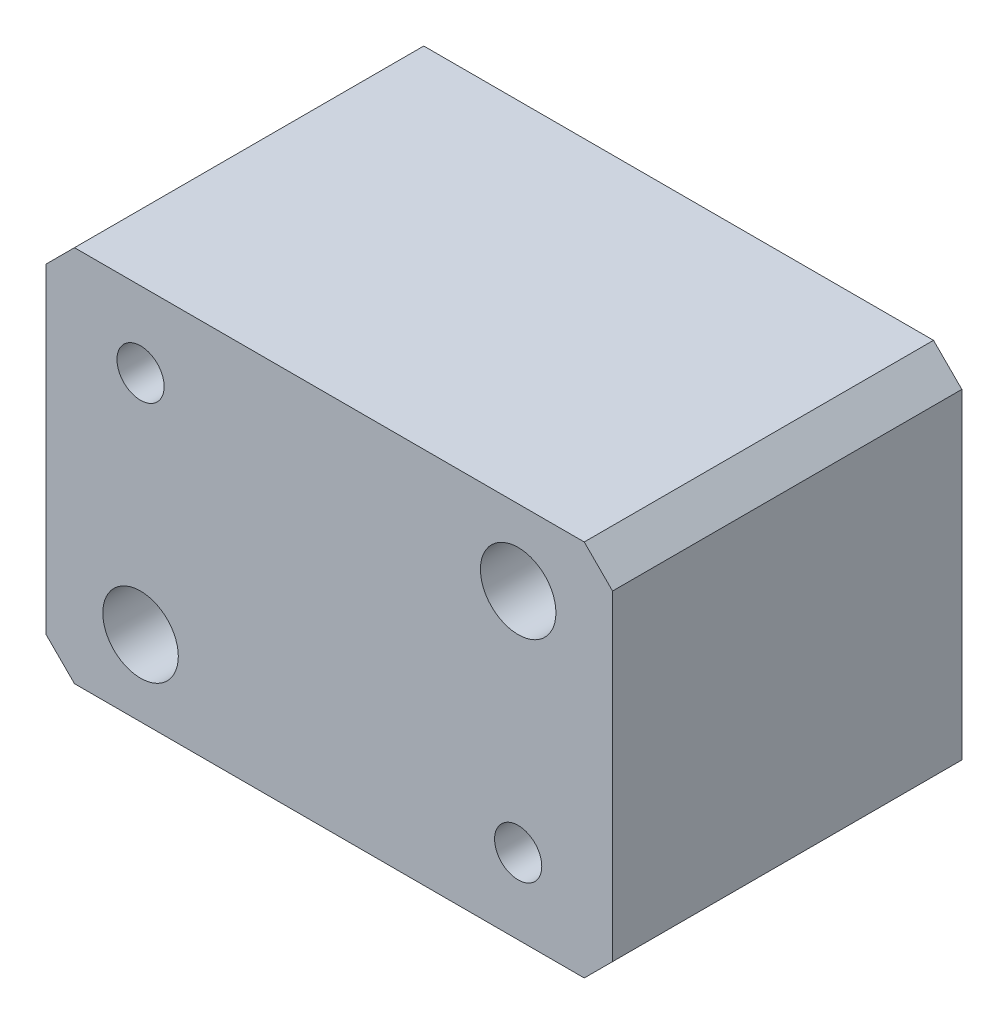
from build123d import *

# Parameters (mm, degrees)
SKETCH1_W                   = 60
SKETCH1_H                   = 40
BOSS_EXTRUDE1_DEPTH         = 37
CHAMFER1_SIZE               = 3
M6_TAPPED_HOLE1_D           = 5
M6_TAPPED_HOLE1_DEPTH       = 12
M6_TAPPED_HOLE1_TIP         = 1.502151548
HOLE1_D                     = 8
HOLE1_DEPTH                 = 10
HOLE2_D                     = 8
HOLE2_DEPTH                 = 10
M6_TAPPED_HOLE2_D           = 5
M6_TAPPED_HOLE2_DEPTH       = 12
M6_TAPPED_HOLE2_CSINK_D     = 6.05
M6_TAPPED_HOLE2_CSINK_ANGLE = 90
M6_TAPPED_HOLE2_TIP         = 1.502151548


with BuildPart() as part:
    # Sketch1 → Boss-Extrude1 (new body)
    with BuildSketch(Plane.XY):
        with Locations((-4.502067899, 30.192307692)):
            Rectangle(SKETCH1_W, SKETCH1_H)
    extrude(amount=BOSS_EXTRUDE1_DEPTH)

    # Chamfer1
    chamfer1_edges = [part.edges().sort_by_distance(p)[0] for p in [
        (-34.502067899, 50.192307692, 18.5),
        (25.497932101, 50.192307692, 18.5),
        (25.497932101, 10.192307692, 18.5),
        (-34.502067899, 10.192307692, 18.5),
    ]]
    chamfer(chamfer1_edges, length=CHAMFER1_SIZE)

    # M6 Tapped Hole1
    with Locations(Plane.XY.offset(37)):
        with Locations((-24.502067899, 42.192307692), (15.497932101, 18.192307692)):
            Hole(M6_TAPPED_HOLE1_D / 2, depth=M6_TAPPED_HOLE1_DEPTH)
            with Locations((0, 0, -(M6_TAPPED_HOLE1_DEPTH + M6_TAPPED_HOLE1_TIP / 2))):  # 118° drill point
                Cone(0, M6_TAPPED_HOLE1_D / 2, M6_TAPPED_HOLE1_TIP, mode=Mode.SUBTRACT)

    # Hole1
    with Locations(Plane.XY.offset(37)):
        with Locations((15.497932101, 42.192307692), (-24.502067899, 18.192307692)):
            Hole(HOLE1_D / 2, depth=HOLE1_DEPTH)

    # Hole2
    with Locations(Plane(origin=(0, 0, 0), x_dir=(-1, 0, 0), z_dir=(0, 0, -1))):
        with Locations((24.502067899, 42.192307692), (-15.497932101, 18.192307692)):
            Hole(HOLE2_D / 2, depth=HOLE2_DEPTH)

    # M6 Tapped Hole2
    with Locations(Plane(origin=(0, 0, 0), x_dir=(-1, 0, 0), z_dir=(0, 0, -1))):
        with Locations((-15.497932101, 42.192307692), (24.502067899, 18.192307692)):
            CounterSinkHole(M6_TAPPED_HOLE2_D / 2, M6_TAPPED_HOLE2_CSINK_D / 2, depth=M6_TAPPED_HOLE2_DEPTH, counter_sink_angle=M6_TAPPED_HOLE2_CSINK_ANGLE)
            with Locations((0, 0, -(M6_TAPPED_HOLE2_DEPTH + M6_TAPPED_HOLE2_TIP / 2))):  # 118° drill point
                Cone(0, M6_TAPPED_HOLE2_D / 2, M6_TAPPED_HOLE2_TIP, mode=Mode.SUBTRACT)


solid = part.part
